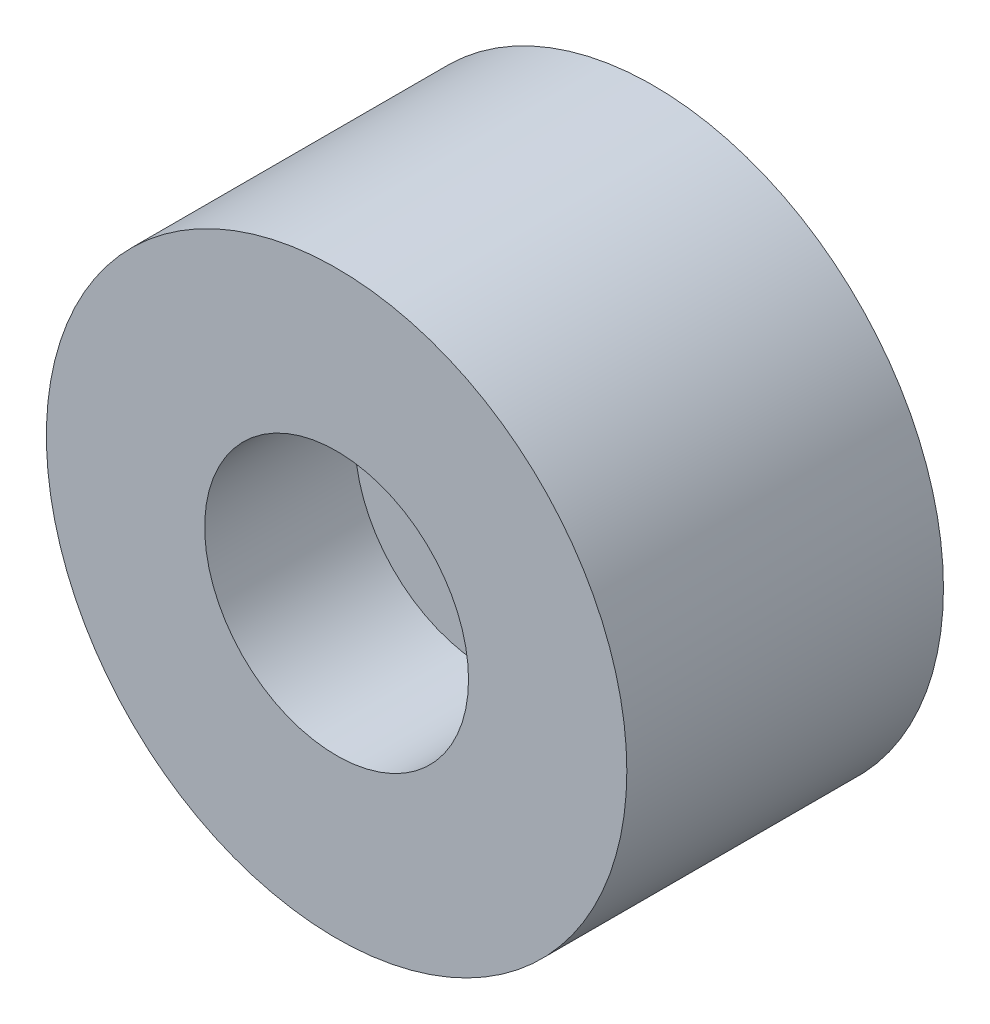
SolidWorks part; units mm, degrees
ref_plane "前视基准面" through (0, 0, 0) normal (0, 0, 1) x (1, 0, 0)
ref_plane "上视基准面" through (0, 0, 0) normal (0, 1, 0) x (1, 0, 0)
ref_plane "右视基准面" through (0, 0, 0) normal (1, 0, 0) x (0, 0, -1)
sketch "草图1" plane through (0, 0, 0) normal (0, 0, 1) x (1, 0, 0)
  circle A0 centre (0, 0) radius 11
  dimension "D1" = 22
extrude "凸台-拉伸1" add sketch "草图1" along normal blind 12
hole_wizard "打孔尺寸(%根据)内六角圆柱头螺钉的类型1" positions "3D草图1" profile "草图2" counterbore size "M5" standard "GB" end condition up to next
sketch3d "3D草图1"
  circle A0 centre (0, 0, 12) radius 11 construction
  point P0 (0, 0, 12)
  point P7 (0, 0, 23)
sketch "草图2" plane through (0, 0, 12) normal (1, 0, 0) x (0, -1, 0)
  line L0 (0, 0) -> (0, 12)
  line L1 (0, 12) -> (2.75, 12)
  line L3 (2.75, 12) -> (2.75, 5.7)
  line L4 (2.75, 5.7) -> (5, 5.7)
  line L5 (5, 5.7) -> (5, 0)
  line L7 (5, 0) -> (0, 0)
  line L11 (0, -6.35) -> (0, 107.95) construction
  dimension "通孔孔直径" = 5.5
  dimension "通孔孔深度" = 12
  dimension "柱形沉头孔直径" = 10
  dimension "柱形沉头孔深度" = 5.7
